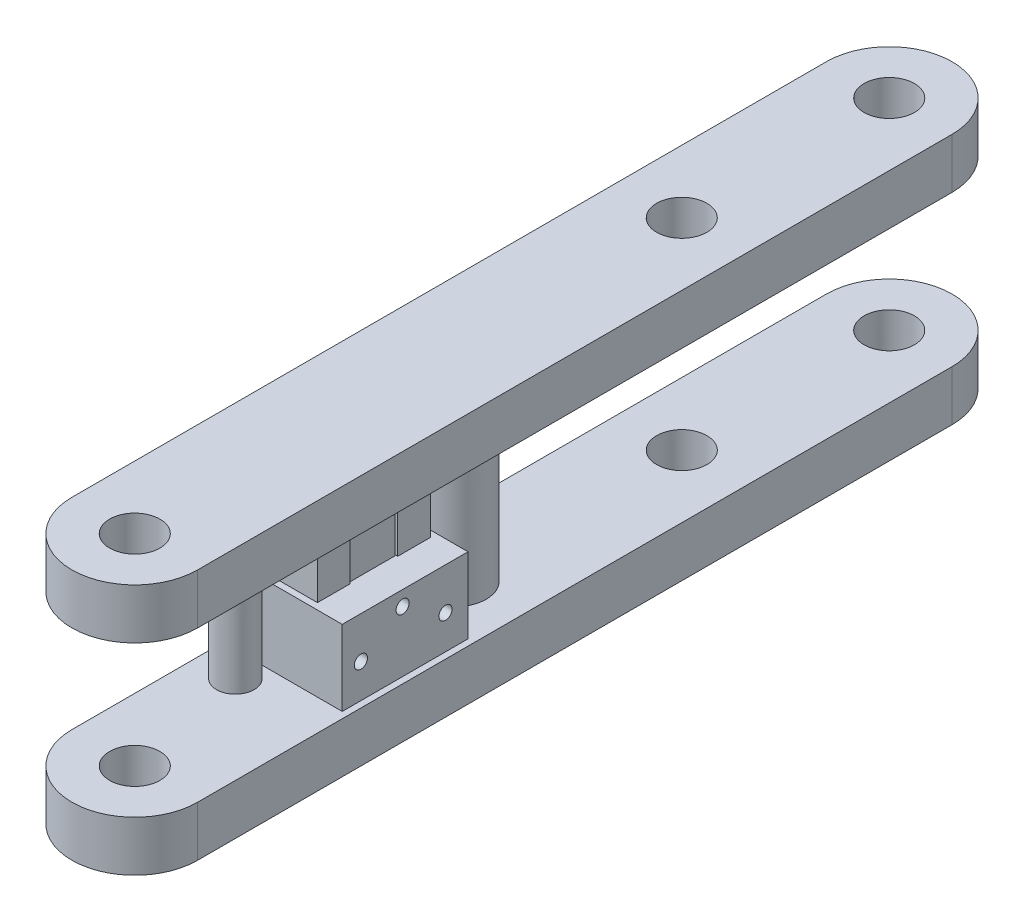
SolidWorks part; units mm, degrees
ref_plane "Front Plane" through (0, 0, 0) normal (0, 0, 1) x (1, 0, 0)
ref_plane "Top Plane" through (0, 0, 0) normal (0, 1, 0) x (1, 0, 0)
ref_plane "Right Plane" through (0, 0, 0) normal (1, 0, 0) x (0, 0, -1)
other "Configuration Table"
sketch "Sketch1" plane through (0, 0, 0) normal (0, 1, 0) x (1, 0, 0)
  line L0 (-5, 0) -> (-5, -60)
  line L1 (0, -0.4726) -> (0, -37.1924) construction
  line L2 (5, 0) -> (5, -60)
  arc A0 (5, 0) -> (-5, 0) centre (0, 0) ccw
  arc A1 (-5, -60) -> (5, -60) centre (0, -60) ccw
  dimension "D1" = 10
  dimension "D3" = 10
  dimension "D2" = 60
extrude "Boss-Extrude1" add sketch "Sketch1" along normal blind 20
sketch "Sketch2" plane through (0, 20, 0) normal (0, 1, 0) x (1, 0, 0)
  line L0 (0, 0) -> (0, -46.0273) construction
  circle A0 centre (0, 0) radius 2
  circle A1 centre (0, -16.5) radius 2
  dimension "D1" = 4
  dimension "D2" = 4
  dimension "D3" = 16.5
extrude "Cut-Extrude1" cut sketch "Sketch2" against normal through all
sketch "Sketch3" plane through (5, 0, 0) normal (1, 0, 0) x (0, 0, -1)
  line L0 (-65, 16) -> (5, 16)
  line L1 (-65, 20) -> (-65, 0) construction
  line L2 (5, 0) -> (5, 20) construction
  line L3 (5, 16) -> (5, 4)
  line L4 (5, 4) -> (-65, 4)
  line L5 (-65, 4) -> (-65, 16)
  line L6 (-60, 20) -> (0, 20) construction
  line L7 (-60, 0) -> (0, 0) construction
  dimension "D1" = 4
  dimension "D2" = 4
extrude "Cut-Extrude2" cut sketch "Sketch3" against normal through all both and the other way through all
sketch "Sketch4" plane through (0, 20, 0) normal (0, 1, 0) x (1, 0, 0)
  circle A0 centre (0, -60) radius 2
  dimension "D1" = 4
extrude "Cut-Extrude3" cut sketch "Sketch4" against normal through all both and the other way through all
sketch "Sketch5" plane through (0, 20, 0) normal (0, 1, 0) x (1, 0, 0)
  circle A0 centre (0, -34.5524) radius 2.5
  dimension "D1" = 5
extrude "Boss-Extrude2" add sketch "Sketch5" against normal up to surface (16 mm away) up to face at (0, 4, 58)
sketch "Sketch6" plane through (0, 20, 0) normal (0, 1, 0) x (1, 0, 0)
  circle A0 centre (-2, -50) radius 1.5
  dimension "D1" = 3
  dimension "D3" = 2
  dimension "D2" = 50
extrude "Boss-Extrude3" add sketch "Sketch6" against normal up to surface (16 mm away) up to face at (0, 4, 32.0524)
sketch "Sketch7" plane through (0, 20, 0) normal (0, 1, 0) x (1, 0, 0)
  line L0 (4.5, -38) -> (-4, -38)
  line L1 (-4, -38) -> (-4, -48)
  line L2 (-4, -48) -> (4.5, -48)
  line L3 (4.5, -48) -> (4.5, -44)
  line L7 (4.5, -44) -> (4.5, -38)
  line L8 (5, -60) -> (5, 0) construction
  circle A0 centre (0, -60) radius 2 construction
  dimension "D1" = 0.5
  dimension "D2" = 9
  dimension "D4" = 10
  dimension "D5" = 12
  dimension "D7" = 4
extrude "Boss-Extrude4" add sketch "Sketch7" along normal blind 6 from surface at -16 starting at face at (-2, 4, 48.5)
sketch "Sketch8" plane through (4.5, 0, 0) normal (1, 0, 0) x (0, 0, -1)
  circle A0 centre (-39.7885, 6.6919) radius 0.5233
  circle A1 centre (-46.5159, 6.6919) radius 0.5233
  circle A2 centre (-43.1996, 8.8238) radius 0.5233
extrude "Cut-Extrude4" cut sketch "Sketch8" against normal through all both and the other way through all
sketch "Sketch9" plane through (0, 10, 0) normal (0, 1, 0) x (1, 0, 0)
  line L0 (0.25, -41.2007) -> (0.25, -38) construction
  line L1 (-1.381, -41.2007) -> (1.881, -41.2007)
  line L2 (-1.381, -41.2007) -> (-1.381, -44.7993)
  line L3 (-1.381, -44.7993) -> (1.881, -44.7993)
  line L4 (1.881, -41.2007) -> (1.881, -44.7993)
  line L5 (-4, -38) -> (4.5, -38) construction
  line L6 (1.881, -43) -> (4.5, -43) construction
  line L7 (4.5, -38) -> (4.5, -48) construction
extrude "Boss-Extrude5" add sketch "Sketch9" along normal blind 4
sketch "Sketch10" plane through (0, 10, 0) normal (0, 1, 0) x (1, 0, 0)
  line L0 (4.5, -43) -> (2.4274, -43) construction
  line L1 (-1.6834, -38.5093) -> (2.0199, -38.5093)
  line L2 (-1.6834, -38.5093) -> (-1.6834, -41.1062)
  line L3 (-1.6834, -41.1062) -> (2.0199, -41.1062)
  line L4 (2.0199, -38.5093) -> (2.0199, -41.1062)
  line L5 (4.5, -38) -> (4.5, -48) construction
  line L6 (2.0199, -47.4907) -> (2.0199, -44.8938)
  line L7 (-1.6834, -44.8938) -> (2.0199, -44.8938)
  line L8 (-1.6834, -47.4907) -> (-1.6834, -44.8938)
  line L9 (-1.6834, -47.4907) -> (2.0199, -47.4907)
extrude "Boss-Extrude6" add sketch "Sketch10" along normal up to surface (6 mm away) up to face at (-2, 16, 51.5)
